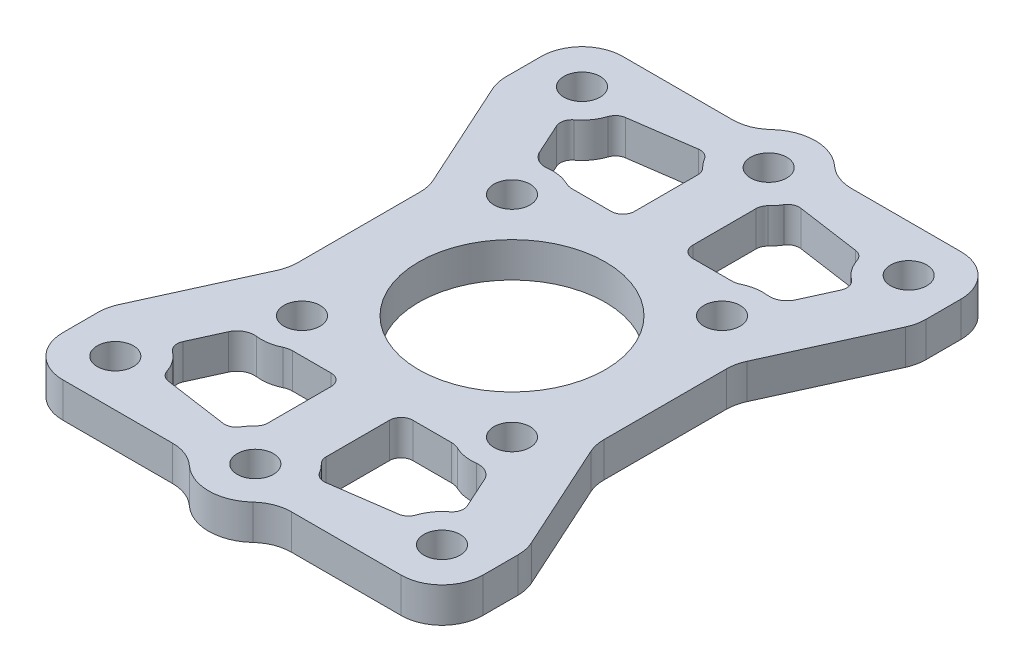
from build123d import *

# Parameters (mm, degrees)
SKETCH_3_R               = 1.55
SKETCH_3_R_2             = 8
EXTRUDE_1_DEPTH          = 3
CUT_EXTRUDE_1_DEPTH      = 32.764760349
CUT_EXTRUDE_1_DEPTH_BACK = 32.764760349
FILLET_1_R               = 3.5
FILLET_6_R               = 1
FILLET_7_R               = 1.5


with BuildPart() as part:
    # 草图3 → 凸台-拉伸1 (new body)
    # profile 1 of 7: a face of its own
    with BuildSketch(Plane(origin=(0, 0, 0), x_dir=(1, 0, 0), z_dir=(0, 1, 0))):
        with BuildLine():
            Line((-18, 24), (-18, -24))
            Line((-18, -24), (-3.464101615, -24))
            ThreePointArc((-3.464101615, -24), (-1.03527618, -18.136296695), (4, -22))
            ThreePointArc((4, -22), (3.863703305, -23.03527618), (3.464101615, -24))
            Line((3.464101615, -24), (18, -24))
            Line((18, -24), (18, 24))
            Line((18, 24), (3.464101615, 24))
            ThreePointArc((3.464101615, 24), (3.863703305, 23.03527618), (4, 22))
            ThreePointArc((4, 22), (-1.03527618, 18.136296695), (-3.464101615, 24))
            Line((-3.464101615, 24), (-18, 24))
        make_face()
        with Locations(Location((-14, -20, 0), (0, 0, 270))):
            Circle(SKETCH_3_R, mode=Mode.SUBTRACT)
        with Locations(Location((-9, -9, 0), (0, 0, 270))):
            Circle(SKETCH_3_R, mode=Mode.SUBTRACT)
        with Locations(Location((14, -20, 0), (0, 0, 270))):
            Circle(SKETCH_3_R, mode=Mode.SUBTRACT)
        with Locations(Location((9, -9, 0), (0, 0, 270))):
            Circle(SKETCH_3_R, mode=Mode.SUBTRACT)
        with Locations(Location((-9, 9, 0), (0, 0, 270))):
            Circle(SKETCH_3_R, mode=Mode.SUBTRACT)
        with Locations(Location((0, 0, 0), (0, 0, 270))):
            Circle(SKETCH_3_R_2, mode=Mode.SUBTRACT)
        with Locations(Location((-14, 20, 0), (0, 0, 270))):
            Circle(SKETCH_3_R, mode=Mode.SUBTRACT)
        with Locations(Location((9, 9, 0), (0, 0, 270))):
            Circle(SKETCH_3_R, mode=Mode.SUBTRACT)
        with Locations(Location((14, 20, 0), (0, 0, 270))):
            Circle(SKETCH_3_R, mode=Mode.SUBTRACT)
    # profile 2 of 7: a face of its own
    with BuildSketch(Plane(origin=(0, 0, 0), x_dir=(1, 0, 0), z_dir=(0, 1, 0))):
        with BuildLine():
            Line((-18, 24), (-18, -24))
            Line((-18, -24), (-3.464101615, -24))
            ThreePointArc((-3.464101615, -24), (-1.03527618, -18.136296695), (4, -22))
            ThreePointArc((4, -22), (3.863703305, -23.03527618), (3.464101615, -24))
            Line((3.464101615, -24), (18, -24))
            Line((18, -24), (18, 24))
            Line((18, 24), (3.464101615, 24))
            ThreePointArc((3.464101615, 24), (3.863703305, 23.03527618), (4, 22))
            ThreePointArc((4, 22), (-1.03527618, 18.136296695), (-3.464101615, 24))
            Line((-3.464101615, 24), (-18, 24))
        make_face()
        with Locations(Location((-14, -20, 0), (0, 0, 270))):
            Circle(SKETCH_3_R, mode=Mode.SUBTRACT)
        with Locations(Location((-9, -9, 0), (0, 0, 270))):
            Circle(SKETCH_3_R, mode=Mode.SUBTRACT)
        with Locations(Location((14, -20, 0), (0, 0, 270))):
            Circle(SKETCH_3_R, mode=Mode.SUBTRACT)
        with Locations(Location((9, -9, 0), (0, 0, 270))):
            Circle(SKETCH_3_R, mode=Mode.SUBTRACT)
        with Locations(Location((-9, 9, 0), (0, 0, 270))):
            Circle(SKETCH_3_R, mode=Mode.SUBTRACT)
        with Locations(Location((0, 0, 0), (0, 0, 270))):
            Circle(SKETCH_3_R_2, mode=Mode.SUBTRACT)
        with Locations(Location((-14, 20, 0), (0, 0, 270))):
            Circle(SKETCH_3_R, mode=Mode.SUBTRACT)
        with Locations(Location((9, 9, 0), (0, 0, 270))):
            Circle(SKETCH_3_R, mode=Mode.SUBTRACT)
        with Locations(Location((14, 20, 0), (0, 0, 270))):
            Circle(SKETCH_3_R, mode=Mode.SUBTRACT)
    # profile 3 of 7: a face of its own
    with BuildSketch(Plane(origin=(0, 0, 0), x_dir=(1, 0, 0), z_dir=(0, 1, 0))):
        with BuildLine():
            Line((-18, 24), (-18, -24))
            Line((-18, -24), (-3.464101615, -24))
            ThreePointArc((-3.464101615, -24), (-1.03527618, -18.136296695), (4, -22))
            ThreePointArc((4, -22), (3.863703305, -23.03527618), (3.464101615, -24))
            Line((3.464101615, -24), (18, -24))
            Line((18, -24), (18, 24))
            Line((18, 24), (3.464101615, 24))
            ThreePointArc((3.464101615, 24), (3.863703305, 23.03527618), (4, 22))
            ThreePointArc((4, 22), (-1.03527618, 18.136296695), (-3.464101615, 24))
            Line((-3.464101615, 24), (-18, 24))
        make_face()
        with Locations(Location((-14, -20, 0), (0, 0, 270))):
            Circle(SKETCH_3_R, mode=Mode.SUBTRACT)
        with Locations(Location((-9, -9, 0), (0, 0, 270))):
            Circle(SKETCH_3_R, mode=Mode.SUBTRACT)
        with Locations(Location((14, -20, 0), (0, 0, 270))):
            Circle(SKETCH_3_R, mode=Mode.SUBTRACT)
        with Locations(Location((9, -9, 0), (0, 0, 270))):
            Circle(SKETCH_3_R, mode=Mode.SUBTRACT)
        with Locations(Location((-9, 9, 0), (0, 0, 270))):
            Circle(SKETCH_3_R, mode=Mode.SUBTRACT)
        with Locations(Location((0, 0, 0), (0, 0, 270))):
            Circle(SKETCH_3_R_2, mode=Mode.SUBTRACT)
        with Locations(Location((-14, 20, 0), (0, 0, 270))):
            Circle(SKETCH_3_R, mode=Mode.SUBTRACT)
        with Locations(Location((9, 9, 0), (0, 0, 270))):
            Circle(SKETCH_3_R, mode=Mode.SUBTRACT)
        with Locations(Location((14, 20, 0), (0, 0, 270))):
            Circle(SKETCH_3_R, mode=Mode.SUBTRACT)
    # profile 4 of 7: a face of its own
    with BuildSketch(Plane(origin=(0, 0, 0), x_dir=(1, 0, 0), z_dir=(0, 1, 0))):
        with BuildLine():
            Line((3.464101615, 24), (-3.464101615, 24))
            ThreePointArc((-3.464101615, 24), (-1.03527618, 18.136296695), (4, 22))
            ThreePointArc((4, 22), (3.863703305, 23.03527618), (3.464101615, 24))
        make_face()
        with Locations(Location((0, 22, 0), (0, 0, 270))):
            Circle(SKETCH_3_R, mode=Mode.SUBTRACT)
    # profile 5 of 7: a face of its own
    with BuildSketch(Plane(origin=(0, 0, 0), x_dir=(1, 0, 0), z_dir=(0, 1, 0))):
        with BuildLine():
            ThreePointArc((3.464101615, 24), (0, 26), (-3.464101615, 24))
            Line((-3.464101615, 24), (3.464101615, 24))
        make_face()
    # profile 6 of 7: a face of its own
    with BuildSketch(Plane(origin=(0, 0, 0), x_dir=(1, 0, 0), z_dir=(0, 1, 0))):
        with BuildLine():
            Line((3.464101615, -24), (-3.464101615, -24))
            ThreePointArc((-3.464101615, -24), (0, -26), (3.464101615, -24))
        make_face()
    # profile 7 of 7: a face of its own
    with BuildSketch(Plane(origin=(0, 0, 0), x_dir=(1, 0, 0), z_dir=(0, 1, 0))):
        with BuildLine():
            ThreePointArc((4, -22), (-1.03527618, -18.136296695), (-3.464101615, -24))
            Line((-3.464101615, -24), (3.464101615, -24))
            ThreePointArc((3.464101615, -24), (3.863703305, -23.03527618), (4, -22))
        make_face()
        with Locations(Location((0, -22, 0), (0, 0, 270))):
            Circle(SKETCH_3_R, mode=Mode.SUBTRACT)
    extrude(amount=EXTRUDE_1_DEPTH)

    # 草图4 → 切除-拉伸1 (cut, two sides: drawn at the far end of the back side and taken through both)
    with BuildSketch(Plane(origin=(0, 3, 0), x_dir=(1, 0, 0), z_dir=(0, 1, 0)).offset(-CUT_EXTRUDE_1_DEPTH_BACK)):
        with BuildLine():
            Line((-12.551689695, 16.813717329), (-10.448310305, 12.186282671))
            ThreePointArc((-10.448310305, 12.186282671), (-8.799783301, 12.494268632), (-7.197224362, 12))
            Line((-7.197224362, 12), (-2.5, 12))
            Line((-2.5, 12), (-2.5, 18.877501001))
            ThreePointArc((-2.5, 18.877501001), (-3.19610794, 19.594819334), (-3.692636546, 20.462327949))
            Line((-3.692636546, 20.462327949), (-10.538187101, 19.484392155))
            ThreePointArc((-10.538187101, 19.484392155), (-11.205281145, 17.892976858), (-12.551689695, 16.813717329))
        make_face()
        with BuildLine():
            Line((2.5, 18.877501001), (2.5, 12))
            Line((2.5, 12), (7.197224362, 12))
            ThreePointArc((7.197224362, 12), (8.799783301, 12.494268632), (10.448310305, 12.186282671))
            Line((10.448310305, 12.186282671), (12.551689695, 16.813717329))
            ThreePointArc((12.551689695, 16.813717329), (11.205281145, 17.892976858), (10.538187101, 19.484392155))
            Line((10.538187101, 19.484392155), (3.692636546, 20.462327949))
            ThreePointArc((3.692636546, 20.462327949), (3.19610794, 19.594819334), (2.5, 18.877501001))
        make_face()
        Polygon((-13.128657261, 6), (-18, 16.716954026), (-18, -16.716954026), (-13.128657261, -6), align=None)
        Polygon((18, -16.716954026), (18, 16.716954026), (13.128657261, 6), (13.128657261, -6), align=None)
        with BuildLine():
            Line((-10.538187101, -19.484392155), (-3.692636546, -20.462327949))
            ThreePointArc((-3.692636546, -20.462327949), (-3.19610794, -19.594819334), (-2.5, -18.877501001))
            Line((-2.5, -18.877501001), (-2.5, -12))
            Line((-2.5, -12), (-7.197224362, -12))
            ThreePointArc((-7.197224362, -12), (-8.799783301, -12.494268632), (-10.448310305, -12.186282671))
            Line((-10.448310305, -12.186282671), (-12.551689695, -16.813717329))
            ThreePointArc((-12.551689695, -16.813717329), (-11.205281145, -17.892976858), (-10.538187101, -19.484392155))
        make_face()
        with BuildLine():
            ThreePointArc((2.5, -18.877501001), (3.19610794, -19.594819334), (3.692636546, -20.462327949))
            Line((3.692636546, -20.462327949), (10.538187101, -19.484392155))
            ThreePointArc((10.538187101, -19.484392155), (11.205281145, -17.892976858), (12.551689695, -16.813717329))
            Line((12.551689695, -16.813717329), (10.448310305, -12.186282671))
            ThreePointArc((10.448310305, -12.186282671), (8.799783301, -12.494268632), (7.197224362, -12))
            Line((7.197224362, -12), (2.5, -12))
            Line((2.5, -12), (2.5, -18.877501001))
        make_face()
    extrude(amount=CUT_EXTRUDE_1_DEPTH + CUT_EXTRUDE_1_DEPTH_BACK, mode=Mode.SUBTRACT)

    # 圆角1
    fillet_1_edges = [part.edges().sort_by_distance(p)[0] for p in [
        (13.128657261, 1.5, 6),
        (13.128657261, 1.5, -6),
        (18, 1.5, -16.716954026),
        (18, 1.5, 16.716954026),
        (-18, 1.5, -16.716954026),
        (-13.128657261, 1.5, -6),
        (-13.128657261, 1.5, 6),
        (-18, 1.5, 16.716954026),
        (-18, 1.5, 24),
        (-18, 1.5, -24),
        (-3.464101615, 1.5, -24),
        (3.464101615, 1.5, -24),
        (18, 1.5, -24),
        (18, 1.5, 24),
        (3.464101615, 1.5, 24),
        (-3.464101615, 1.5, 24),
    ]]
    fillet(fillet_1_edges, radius=FILLET_1_R)

    # 圆角6
    fillet_6_edges = [part.edges().sort_by_distance(p)[0] for p in [
        (-12.551689695, 1.5, 16.813717329),
        (-2.5, 1.5, 12),
        (-2.5, 1.5, 18.877501001),
        (-3.692636546, 1.5, 20.462327949),
        (-10.538187101, 1.5, 19.484392155),
        (12.551689695, 1.5, -16.813717329),
        (2.5, 1.5, -12),
        (2.5, 1.5, -18.877501001),
        (3.692636546, 1.5, -20.462327949),
        (10.538187101, 1.5, -19.484392155),
        (2.5, 1.5, 18.877501001),
        (2.5, 1.5, 12),
        (12.551689695, 1.5, 16.813717329),
        (10.538187101, 1.5, 19.484392155),
        (3.692636546, 1.5, 20.462327949),
        (-3.692636546, 1.5, -20.462327949),
        (-2.5, 1.5, -18.877501001),
        (-2.5, 1.5, -12),
        (-12.551689695, 1.5, -16.813717329),
        (-10.538187101, 1.5, -19.484392155),
    ]]
    fillet(fillet_6_edges, radius=FILLET_6_R)

    # 圆角7
    fillet_7_edges = [part.edges().sort_by_distance(p)[0] for p in [
        (-10.448310305, 1.5, 12.186282671),
        (-7.197224362, 1.5, 12),
        (10.448310305, 1.5, -12.186282671),
        (7.197224362, 1.5, -12),
        (7.197224362, 1.5, 12),
        (10.448310305, 1.5, 12.186282671),
        (-7.197224362, 1.5, -12),
        (-10.448310305, 1.5, -12.186282671),
    ]]
    fillet(fillet_7_edges, radius=FILLET_7_R)


solid = part.part
